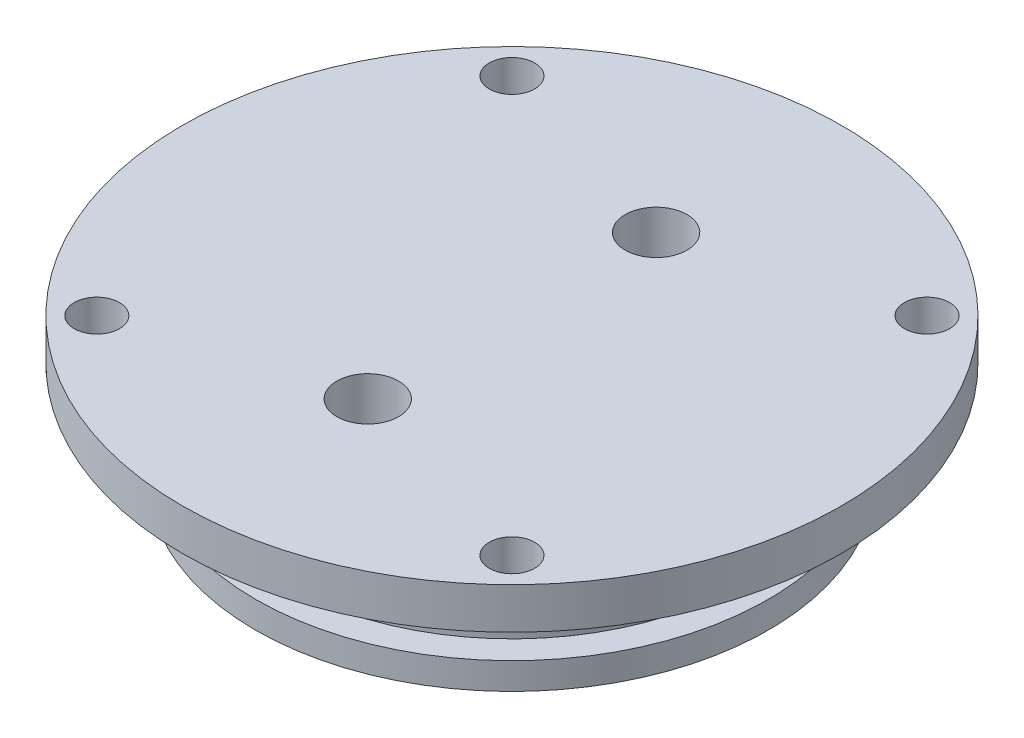
SolidWorks part; units mm, degrees
ref_plane "前视基准面" through (0, 0, 0) normal (0, 0, 1) x (1, 0, 0)
ref_plane "上视基准面" through (0, 0, 0) normal (0, 1, 0) x (1, 0, 0)
ref_plane "右视基准面" through (0, 0, 0) normal (1, 0, 0) x (0, 0, -1)
sketch "草图1" plane through (0, 0, 0) normal (0, 0, 1) x (1, 0, 0)
  line L0 (0, 0) -> (12.45, 0)
  line L5 (12.45, 0) -> (12.45, 1.295)
  line L6 (12.45, 1.295) -> (11.1546, 1.295)
  line L7 (11.1546, 1.295) -> (11.1546, 3.708)
  line L8 (11.1546, 3.708) -> (12.45, 3.708)
  line L9 (12.45, 3.708) -> (12.45, 5)
  line L10 (12.45, 5) -> (16, 5)
  line L11 (16, 5) -> (16, 7)
  line L12 (16, 7) -> (0, 7)
  line L13 (0, 7) -> (0, 0)
revolve "旋转1" add sketch "草图1" angle 360 about L13
hole_wizard "大小mm 暗销孔1" positions "草图4" profile "草图5" hole size "Ø2.0" standard "GB"
sketch "草图4" plane through (0, 7, 0) normal (0, 1, 0) x (1, 0, 0)
  line L1 (-10.0763, 10.0763) -> (0, 0) construction
  line L3 (0, 0) -> (0, 16.852) construction
  point P10 (-10.0763, 10.0763)
  point P27 (10.0763, 10.0763)
  point P28 (10.0763, -10.0763)
  point P29 (-10.0763, -10.0763)
  dimension "D1" = 4
  dimension "D3" = 45
  dimension "D4" = 14.25
sketch "草图5" plane through (-10.0763, 7, 10.0763) normal (1, 0, 0) x (0, 0, 1)
  line L0 (0, 0) -> (0, 7.7609)
  line L1 (0, 7.7609) -> (1.1, 7.1)
  line L2 (1.1, 7.1) -> (1.1, 0)
  line L5 (1.1, 0) -> (0, 0)
  line L10 (0, 7.7609) -> (-1.1, 7.1) construction
  line L11 (0, -6.35) -> (0, 107.95) construction
  dimension "孔直径" = 2.2
  dimension "孔深度" = 7.1
  dimension "导头角度" = 118
sketch "草图7" plane through (0, 0, 0) normal (0, -1, 0) x (1, 0, 0)
  line L0 (0, 7) -> (0, -7) construction
  line L1 (9, 0) -> (-9, 0) construction
  circle A0 centre (-9, 0) radius 2.5
  circle A1 centre (9, 0) radius 2.5
  circle A2 centre (0, -7) radius 1.5
  circle A3 centre (0, 7) radius 1.5
  dimension "D1" = 3
  dimension "D2" = 3
  dimension "D3" = 5
  dimension "D4" = 5
extrude "切除-拉伸1" cut sketch "草图7" against normal blind 5
sketch "草图8" plane through (0, 5, 0) normal (0, -1, 0) x (1, 0, 0)
  circle A1 centre (0, 7) radius 1.5
  circle A2 centre (0, 7) radius 1.5
  circle A3 centre (0, -7) radius 1.5
  circle A4 centre (0, -7) radius 1.5
  dimension "D1" = 0
  dimension "D2" = 0
extrude "切除-拉伸2" cut sketch "草图8" against normal blind 5
